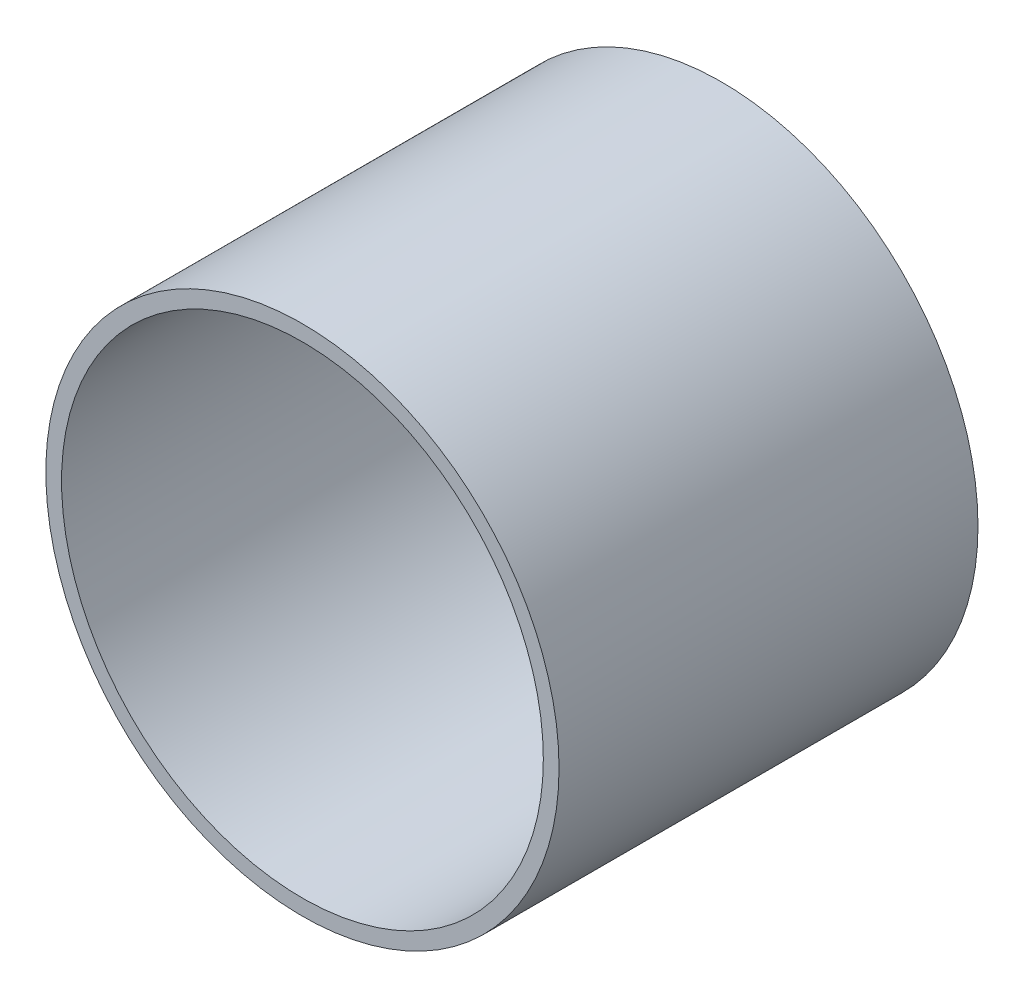
from build123d import *

# Parameters (mm, degrees)
SKETCH_1_R      = 49
SKETCH_1_R_2    = 46
EXTRUDE_1_DEPTH = 40


with BuildPart() as part:
    # 草图1 → 凸台-拉伸1 (new, symmetric)
    with BuildSketch(Plane.XY):
        Circle(SKETCH_1_R)
        Circle(SKETCH_1_R_2, mode=Mode.SUBTRACT)
    extrude(amount=EXTRUDE_1_DEPTH, both=True)


solid = part.part
